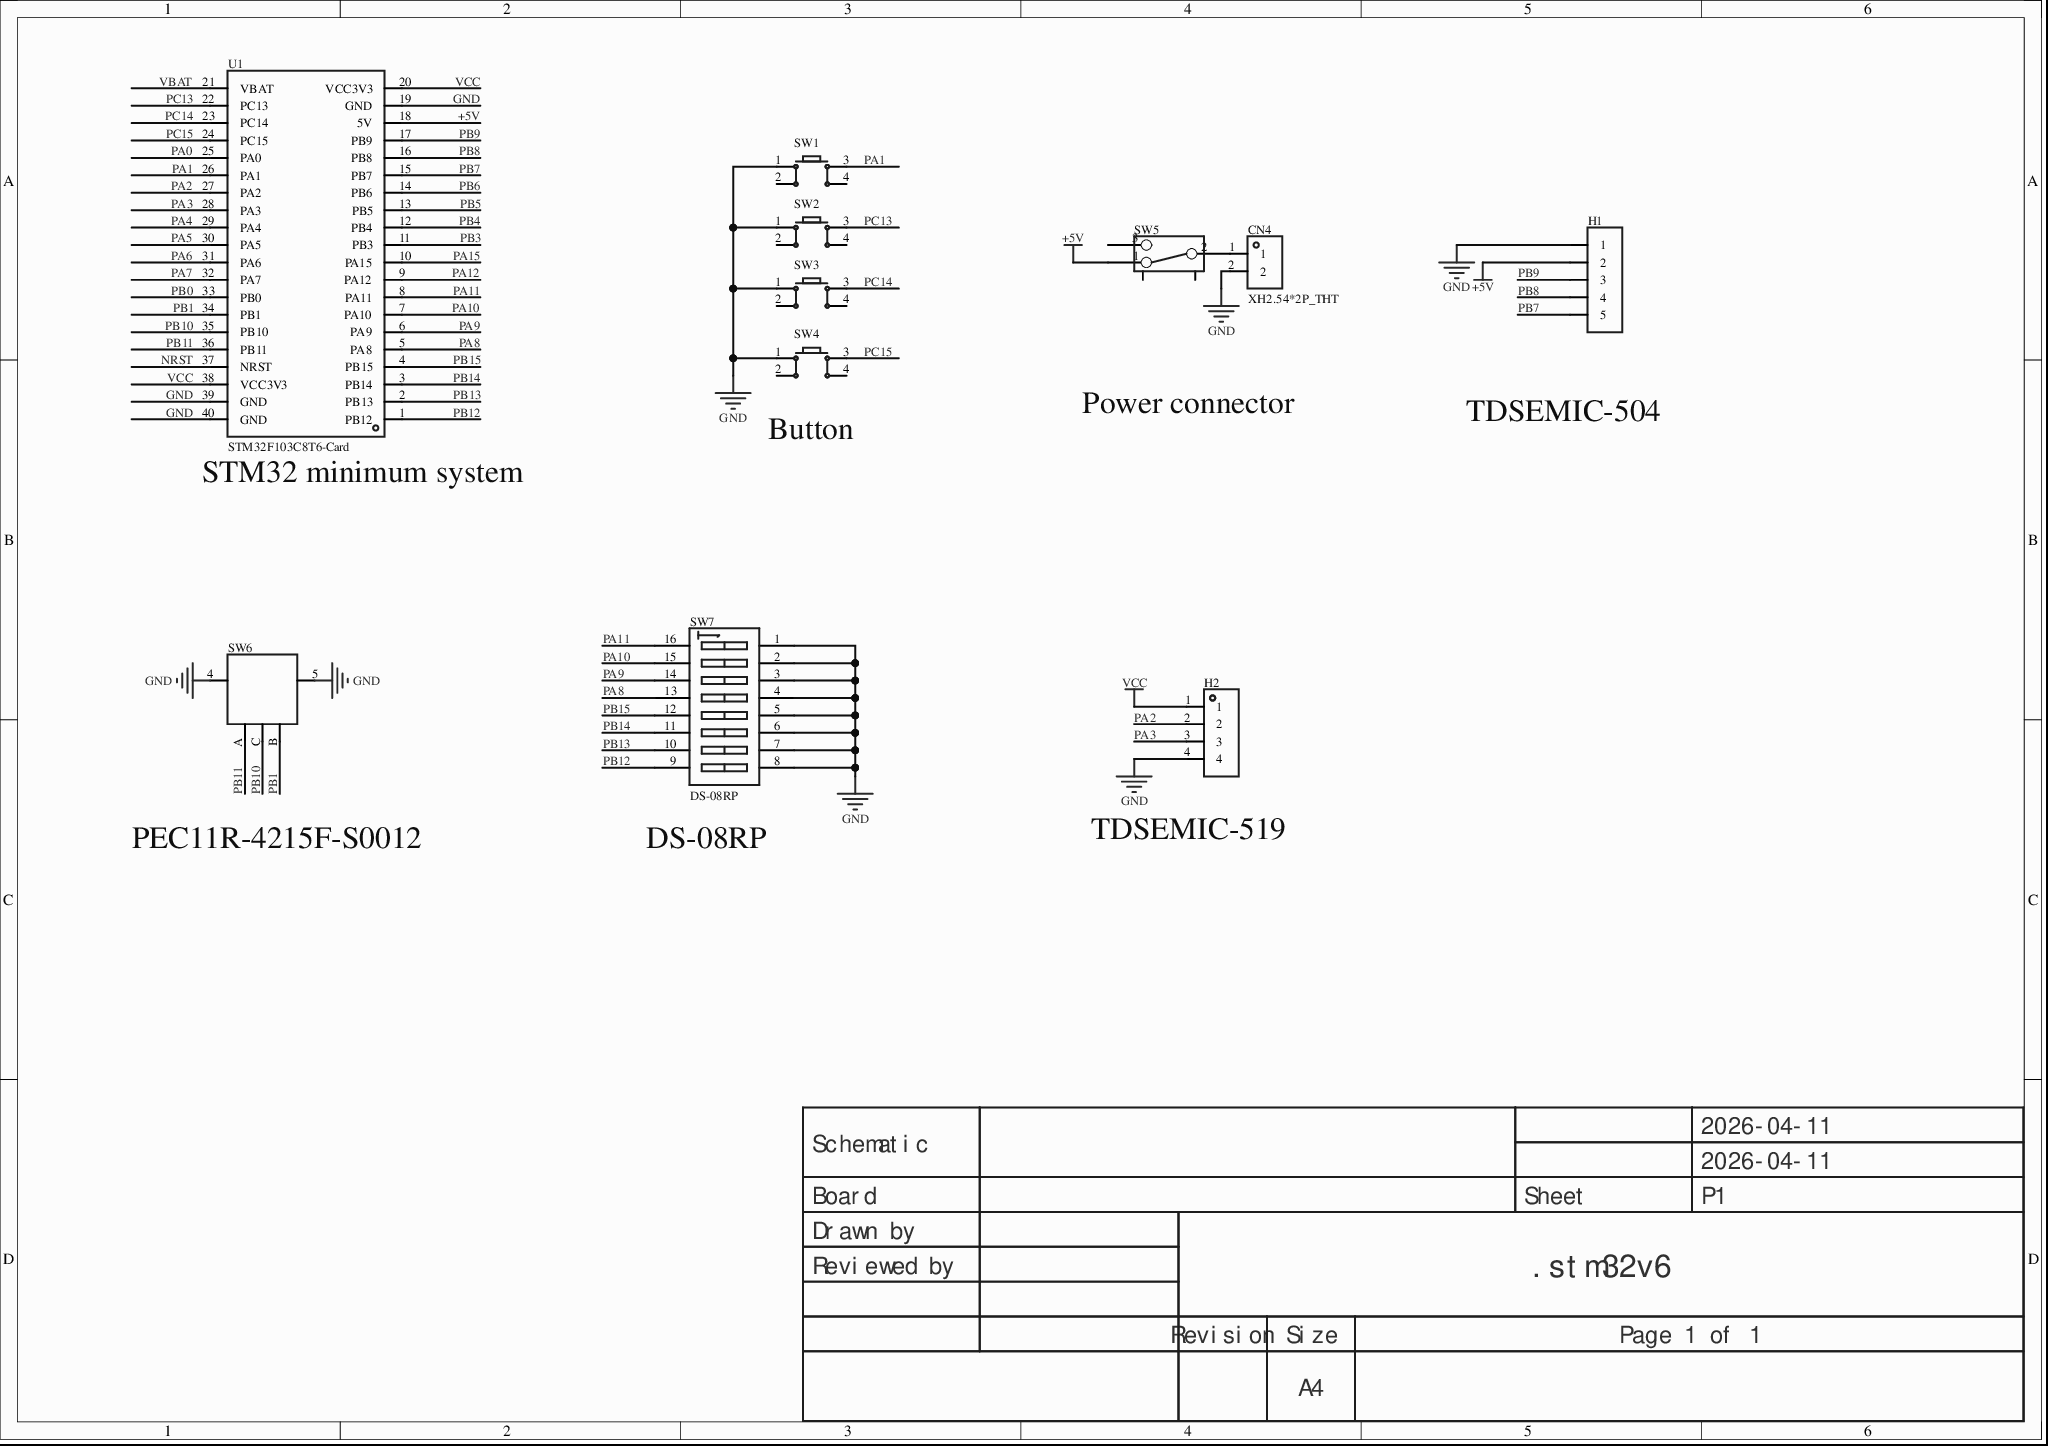
[diagram p0: MISC51872-3.schdoc]
# Altium project MISC51872-2.PrjPcb
1 sheet, 11 parts. Net scope: global (net labels, ports and power ports of the same name join across sheets).
Board file: MISC51872.pcbdoc

## Sheet MISC51872-3.schdoc
size 297 x 209 mm; Version: V1.0; @Project Name: MISC51872; @Page Count: 1; @Update Date: 2026-04-11; @Create Date: 2026-04-11; @Schematic Name: MISC51872; @Page No: 1; @Create Time: 23:22:16; @Update Time: 17:32:40; @Board Name: MISC51872

### Parts
CN4  XH2.54*2P_THT  [CONN-TH_2P-P2.50-XH2.54-2P]
H1  (no value)  [HDR-TH_5P-P2.54-V-F]
H2  (no value)  [HDR-TH_4P-P2.54-V-F]
SW1  (no value)  [SW-TH_4P-L6.0-W6.0-P4.50-LS6.5]
SW2  (no value)  [SW-TH_4P-L6.0-W6.0-P4.50-LS6.5]
SW3  (no value)  [SW-TH_4P-L6.0-W6.0-P4.50-LS6.5]
SW4  (no value)  [SW-TH_4P-L6.0-W6.0-P4.50-LS6.5]
SW5  (no value)  [拨动开关]
SW6  PEC11R-4215F-N0024  [SW-TH_PEC11R-4215F-N0024]  (value not drawn)
SW7  DS-08RP  [SW-TH_DS-08XP]
U1  STM32F103C8T6-Card  [CONN-TH_L53.3-W22.9_STM32F103C8T6-CARD]

### Nets
+5V: H1.2 SW5.1 U1.18(5V)
GND: CN4.2 H1.1 H2.4 SW1.1 SW2.1 SW3.1 SW4.1 SW6.4 SW6.5 SW7.1(A1) SW7.2(A2) SW7.3(A3) SW7.4(A4) SW7.5(A5) SW7.6(A6) SW7.7(A7) SW7.8(A8) U1.19(GND) U1.39(GND) U1.40(GND)
VCC: H2.1 U1.20(VCC3V3) U1.38(VCC3V3)
NRST: U1.37(NRST)
PA0: U1.25(PA0)
PA1: SW1.3 U1.26(PA1)
PA2: H2.2 U1.27(PA2)
PA3: H2.3 U1.28(PA3)
PA4: U1.29(PA4)
PA5: U1.30(PA5)
PA6: U1.31(PA6)
PA7: U1.32(PA7)
PA8: SW7.13 U1.5(PA8)
PA9: SW7.14 U1.6(PA9)
PA10: SW7.15 U1.7(PA10)
PA11: SW7.16 U1.8(PA11)
PA12: U1.9(PA12)
PA15: U1.10(PA15)
PB0: U1.33(PB0)
PB1: SW6.B U1.34(PB1)
PB3: U1.11(PB3)
PB4: U1.12(PB4)
PB5: U1.13(PB5)
PB6: U1.14(PB6)
PB7: H1.5 U1.15(PB7)
PB8: H1.4 U1.16(PB8)
PB9: H1.3 U1.17(PB9)
PB10: SW6.C U1.35(PB10)
PB11: SW6.A U1.36(PB11)
PB12: SW7.9 U1.1(PB12)
PB13: SW7.10 U1.2(PB13)
PB14: SW7.11 U1.3(PB14)
PB15: SW7.12 U1.4(PB15)
PC13: SW2.3 U1.22(PC13)
PC14: SW3.3 U1.23(PC14)
PC15: SW4.3 U1.24(PC15)
VBAT: U1.21(VBAT)
NetCN4_1: CN4.1 SW5.2

Not connected (* = marked no-connect by the designer): SW1 2 4; SW2 2 4; SW3 2 4; SW4 2 4; SW5 3 4 5

### Notes on the sheet
- Power connector
- TDSEMIC-504
- (near U1) STM32 minimum system
- (near SW4) Button
- PEC11R-4215F-S0012
- (near SW7) DS-08RP
- (near H2) TDSEMIC-519
- Labels drawn without touching a wire or pin: VCC
- 2026-04-11
- Schematic
- Board
- Sheet
- P1
- Drawn by
- Reviewed by
- .stm32v6
- Revision
- Size
- A4
- Page 1 of 1

### Library data of the parts
CN4 = XH2.54*2P_直插: 3D Model: 325c595e30db4df8abe76612dd40b0fa0819f05c4eef4c71ace90d822a990e87; 3D Model Transform: 295.275,228.346,0,180,0,0,-0.002,-20.079,-137.795; AddInBom: yes; Symbol: XH2.54*2P_THT; Device: XH2.54*2P_THT; LCSC Part Name: XH2.54*2P_直插; Supplier Part: C9900008615; Manufacturer Part: XH2.54*2P_直插; Supplier Footprint: XH2.54_2P; JLCPCB Part Class: Extended Part; Supplier: LCSC; ConvertToPcb: yes; FootprintName: CONN-TH_2P-P2.50-XH2.54-2P; ModelName: CONN-TH_2P-P2.50-XH2.54-2P
H1 = HDR-F_2.54_1x5P: Symbol: Header-Female-2.54_1x5; ConvertToPcb: yes; ModelId: f49cb6116a3d45e5a64915bf3e00773f; ModelTransform: 519.684,98.464,0,0,0,0,0,0,-124.016; Device: HDR-F_2.54_1x5P; AddInBom: yes; SupplierPart: C50950; Supplier Footprint: 插件; FootprintName: HDR-TH_5P-P2.54-V-F; ModelName: HDR-TH_5P-P2.54-V-F
H2 = HDR-F_2.54_1x4P: Symbol: 2.54-1*4P female; ConvertToPcb: yes; ModelId: d187812051054f85879fcaa51a310d8e0819f05c4eef4c71ace90d822a990e87; ModelTransform: 419.6842,98.464,0,0,0,0,0,0,-118.11; Device: HDR-F_2.54_1x4P; AddInBom: yes; SupplierPart: C2718488; Supplier Footprint: 插件; FootprintName: HDR-TH_4P-P2.54-V-F; ModelName: HDR-TH_4P-P2.54-V-F
SW1-SW4 = Key_TH_6x6x6: Contact current:50mA; Rated voltage (DC):12V; Insulation resistance:100MΩ; Circuit: SPST; Mounting: through-hole; Button shape: round; Button/cap colour: black; Actuation force:260gf@±30gf; Operating temperature:-25℃~+70℃; Pin style: PC pin; Switch length:6mm; Switch width:6mm; Switch height:6mm; With bracket: no;; Symbol: Tact switch; AddInBom: yes; ModelId: 20eee248bc684ccd8cbdbb1d0d91ec6f0819f05c4eef4c71ace90d822a990e87; ModelName: SW-TH_4P-L6.0-W6.0-H5.0-LS6.5-P4.50; ModelTransform: 236.22,323.03,0,90,0,0,0,0,-137.795; Device: Key_TH_6x6x6; ConvertToPcb: yes; FootprintName: SW-TH_4P-L6.0-W6.0-P4.50-LS6.5; Supplier Footprint: 插件
SW5 = 拨动开关_正: Symbol: Toggle switch; Device: Toggle switch_upright; ConvertToPcb: yes; ModelId: 4321fe59a4074cbfb4989553f297c68f0819f05c4eef4c71ace90d822a990e87; ModelName: SW-TH_SS-12D02-VG4; ModelTransform: 370.09,208.7,472.35,0,0,0,0,0,-110; AddInBom: yes; Supplier Footprint: 插件; FootprintName: Toggle switch
SW6 = PEC11R-4215F-N0024: Manufacturer: BOURNS; AddInBom: yes; ModelId: 6e2a81c35bd442dab58b578066ac64950819f05c4eef4c71ace90d822a990e87; ModelTransform: 535.432,527.558,0,0,0,0,0,116.26,-137.795; Symbol: PEC11R-4215F-N0024; Device: PEC11R-4215F-N0024; LCSC Part Name: PEC11R-4215F-N0024; SupplierPart: C143791; ManufacturerPart: PEC11R-4215F-N0024; Supplier Footprint: 插件; JLCPCB Part Class: Extended Part; Datasheet: example.com/datasheet/PEC11R-4215F-N0024/155122.html; Supplier: LCSC; ConvertToPcb: yes; FootprintName: SW-TH_PEC11R-4215F-N0024; ModelName: SW-TH_PEC11R-4215F-N0024
SW7 = DS-08RP: Type: flat toggle, raised; Circuit: SPST; Positions: 8; Rated current:25mA; Rated voltage:24V; Operating life:3 thousand cycles; Colour: red;; Manufacturer: XKB Connection(中国星坤); Symbol: DS-08RP_C319056; AddInBom: yes; ModelId: 738dc420ce6c45258f943fd2d1e35cfe0819f05c4eef4c71ace90d822a990e87; ModelName: SW-TH_DS-08XP-L22.0-W9.6-H6.8-P2.54; ModelTransform: 865.35268,377.952,0,0,0,0,0,0,-129.921; Number of Positions: 8 positions; Current Rating: 25mA; Voltage Rating: 24V; Device: DS-08RP; LCSC Part Name: 间距2.54mm 平拨,凸起式 8位拨码开关; SupplierPart: C319056; ManufacturerPart: DS-08RP; Supplier Footprint: 插件; JLCPCB Part Class: Extended Part; Datasheet: example.com/datasheet/DS-08RP/300148.html; Supplier: LCSC; ConvertToPcb: yes; FootprintName: SW-TH_DS-08XP; Type: Flat toggle, raised; Termination Style: PC pin; Lead Pitch: 2.54mm; Operating Temperature: -20℃~+70℃; Operating Life: 3 thousand cycles; Color: Red
U1 = STM32F103C8T6-Card: AddInBom: yes; Symbol: STM32F103C8T6-CARD; Device: STM32F103C8T6-Card; LCSC Part Name: STM32F103C8T6-Card; SupplierPart: C9900077949; ManufacturerPart: STM32F103C8T6-Card; Supplier Footprint: 插件; Supplier: LCSC; ConvertToPcb: yes; FootprintName: CONN-TH_L53.3-W22.9_STM32F103C8T6-CARD